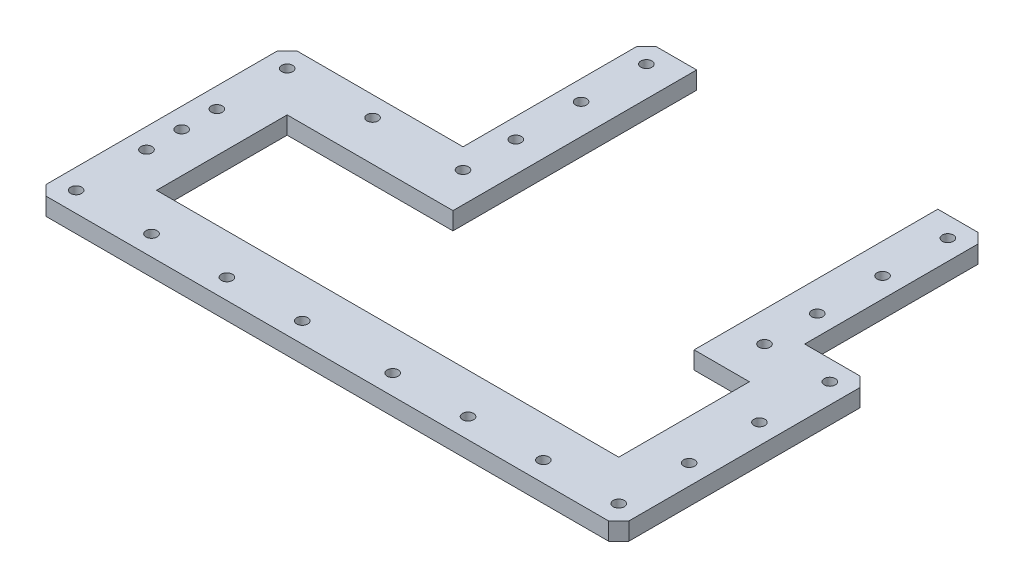
SolidWorks part; units mm, degrees
ref_plane "前视基准面" through (0, 0, 0) normal (0, 0, 1) x (1, 0, 0)
ref_plane "上视基准面" through (0, 0, 0) normal (0, 1, 0) x (1, 0, 0)
ref_plane "右视基准面" through (0, 0, 0) normal (1, 0, 0) x (0, 0, -1)
sketch "草图1" plane through (0, 0, 0) normal (0, 1, 0) x (1, 0, 0)
  line L0 (-1160, 500) -> (-810, 500)
  line L1 (0, 0) -> (-1160, 0)
  line L2 (0, 0) -> (0, 500)
  line L3 (-130, 865) -> (-230, 865)
  line L4 (-1160, 0) -> (-1160, 500)
  line L5 (-810, 500) -> (-810, 865)
  line L6 (-130, 865) -> (-130, 500)
  line L7 (-130, 500) -> (0, 500)
  line L8 (-710, 865) -> (-710, 745)
  line L9 (-470, 1014.2039) -> (-470, -321.2652) construction
  line L10 (-230, 865) -> (-230, 745)
  line L11 (-710, 745) -> (-230, 745)
  line L12 (-710, 865) -> (-810, 865)
  point P15 (-230, 805)
  dimension "D1" = 1160
  dimension "D2" = 500
  dimension "D3" = 365
  dimension "D4" = 100
  dimension "D5" = 100
  dimension "D6" = 450
  dimension "D7" = 230
  dimension "D8" = 120
extrude "凸台-拉伸1" add sketch "草图1" along normal blind 35
sketch "草图4" plane through (0, 35, 0) normal (0, 1, 0) x (1, 0, 0)
  line L18 (-1160, 500) -> (-1160, 0)
  line L19 (-1040, 120) -> (-120, 120)
  line L20 (-1160, 0) -> (0, 0)
  line L21 (-120, 120) -> (-120, 380)
  line L22 (0, 0) -> (0, 500)
  line L23 (-120, 380) -> (-230, 380)
  line L24 (0, 500) -> (-130, 500)
  line L25 (-130, 500) -> (-130, 865)
  line L27 (-130, 865) -> (-230, 865)
  line L28 (-230, 865) -> (-230, 745)
  line L29 (-230, 745) -> (-710, 745)
  line L30 (-710, 745) -> (-710, 865)
  line L31 (-710, 865) -> (-810, 865)
  line L33 (-810, 865) -> (-810, 500)
  line L34 (-810, 500) -> (-1160, 500)
  line L38 (-1160, 0) -> (0, 0)
  line L58 (-710, 380) -> (-1040, 380)
  line L59 (-1040, 380) -> (-1040, 120)
  line L60 (0, 0) -> (0, 500)
  line L61 (0, 500) -> (-130, 500)
  line L62 (-130, 500) -> (-130, 865)
  line L63 (-130, 865) -> (-230, 865)
  line L64 (-230, 865) -> (-230, 745)
  line L65 (-230, 745) -> (-710, 745)
  line L66 (-710, 745) -> (-710, 865)
  line L67 (-710, 865) -> (-810, 865)
  line L68 (-810, 865) -> (-810, 500)
  line L69 (-810, 500) -> (-1160, 500)
  line L70 (-1160, 500) -> (-1160, 0)
  line L71 (-1160, 0) -> (0, 0)
  line L72 (0, 0) -> (0, 500) construction
  line L73 (0, 500) -> (-130, 500) construction
  line L74 (-130, 500) -> (-130, 865) construction
  line L75 (-130, 865) -> (-230, 865) construction
  line L76 (-230, 865) -> (-230, 745) construction
  line L77 (-230, 745) -> (-710, 745) construction
  line L78 (-710, 745) -> (-710, 865) construction
  line L79 (-710, 865) -> (-810, 865) construction
  line L80 (-810, 865) -> (-810, 500) construction
  line L81 (-810, 500) -> (-1160, 500) construction
  line L82 (-1160, 500) -> (-1160, 0) construction
  line L83 (-1160, 0) -> (0, 0) construction
  line L84 (-1040, 120) -> (-120, 120)
  line L85 (-1160, 120) -> (0, 120) construction
  line L86 (-710, 380) -> (-710, 775)
  line L87 (-710, 775) -> (-230, 775)
  line L88 (-230, 775) -> (-230, 380)
  line L89 (-690, 380) -> (-1040, 380) construction
  line L90 (-120, 380) -> (-250, 380) construction
  line L103 (-250, 625) -> (-690, 625) construction
  line L104 (-690, 625) -> (-690, 380) construction
  line L105 (-250, 380) -> (-250, 625) construction
  line L106 (-250, 625) -> (-250, 625) construction
  line L107 (-250, 625) -> (-250, 625) construction
  line L108 (-690, 625) -> (-690, 625) construction
  line L109 (-690, 625) -> (-690, 625) construction
  dimension "D3" = 120
  dimension "D4" = 100
  dimension "D5" = 100
  dimension "D6" = 90
  dimension "D1" = 0
  dimension "D2" = 0
extrude "切除-拉伸1" cut sketch "草图4" against normal through all and the other way through all
sketch "草图5" plane through (0, 35, 0) normal (0, 1, 0) x (1, 0, 0)
  line L0 (-1160, 500) -> (-1160, 0) construction
  line L1 (-1160, 40) -> (0, 40) construction
  line L2 (0, 0) -> (0, 500) construction
  line L3 (-1160, 0) -> (0, 0) construction
  line L4 (-770, 1019.7156) -> (-770, -173.41) construction
  line L5 (-950, 997.2884) -> (-950, -278.8177) construction
  line L6 (-710, 865) -> (-230, 865) construction
  line L7 (-470, 1035.2394) -> (-470, -318.0992) construction
  line L8 (-710, 380) -> (-710, 865) construction
  line L9 (-1120, 997.2884) -> (-1120, -206.0693) construction
  line L10 (-1120, 460) -> (-710, 460) construction
  line L11 (-710, 380) -> (-710, 865) construction
  line L12 (-40, 460) -> (-40, 0) construction
  circle A0 centre (-1120, 40) radius 11
  circle A2 centre (-970, 40) radius 11
  circle A3 centre (-820, 40) radius 11
  circle A4 centre (-670, 40) radius 11
  circle A5 centre (-490, 40) radius 11
  circle A6 centre (-340, 40) radius 11
  circle A7 centre (-190, 40) radius 11
  circle A8 centre (-40, 40) radius 11
  circle A9 centre (-770, 825) radius 11
  circle A10 centre (-770, 695) radius 11
  circle A11 centre (-770, 565) radius 11
  circle A12 centre (-770, 460) radius 11
  circle A13 centre (-1120, 180) radius 11
  circle A14 centre (-1120, 250) radius 11
  circle A15 centre (-1120, 320) radius 11
  circle A16 centre (-1120, 460) radius 11
  circle A17 centre (-950, 460) radius 11
  circle A18 centre (-170, 460) radius 11
  circle A19 centre (-170, 565) radius 11
  circle A20 centre (-170, 695) radius 11
  circle A21 centre (-170, 825) radius 11
  circle A22 centre (-40, 460) radius 11
  circle A23 centre (-40, 320) radius 11
  circle A24 centre (-40, 180) radius 11
  dimension "D1" = 22
  dimension "D5" = 40
  dimension "D8" = 22
  dimension "D14" = 22
  dimension "D2" = 40
  dimension "D4" = 150
  dimension "D6" = 180
  dimension "D9" = 150
  dimension "D10" = 240
  dimension "D11" = 300
  dimension "D12" = 180
  dimension "D13" = 170
  dimension "D15" = 140
  dimension "D16" = 70
  dimension "D17" = 70
  dimension "D18" = 140
  dimension "D19" = 105
  dimension "D20" = 130
  dimension "D21" = 130
  dimension "D22" = 105
  dimension "D23" = 140
  dimension "D24" = 140
  dimension "D25" = 140
  dimension "D26" = 130
  dimension "D27" = 130
  dimension "D3" = 4
  dimension "D7" = 4
chamfer "倒角2" distance 20 angle 45 6 edges at (-1160, 17.5, 0) (0, 17.5, 0) (0, 17.5, -500) (-130, 17.5, -865) (-810, 17.5, -865) (-1160, 17.5, -500)
extrude "切除-拉伸2" cut sketch "草图5" against normal through all both and the other way through all
